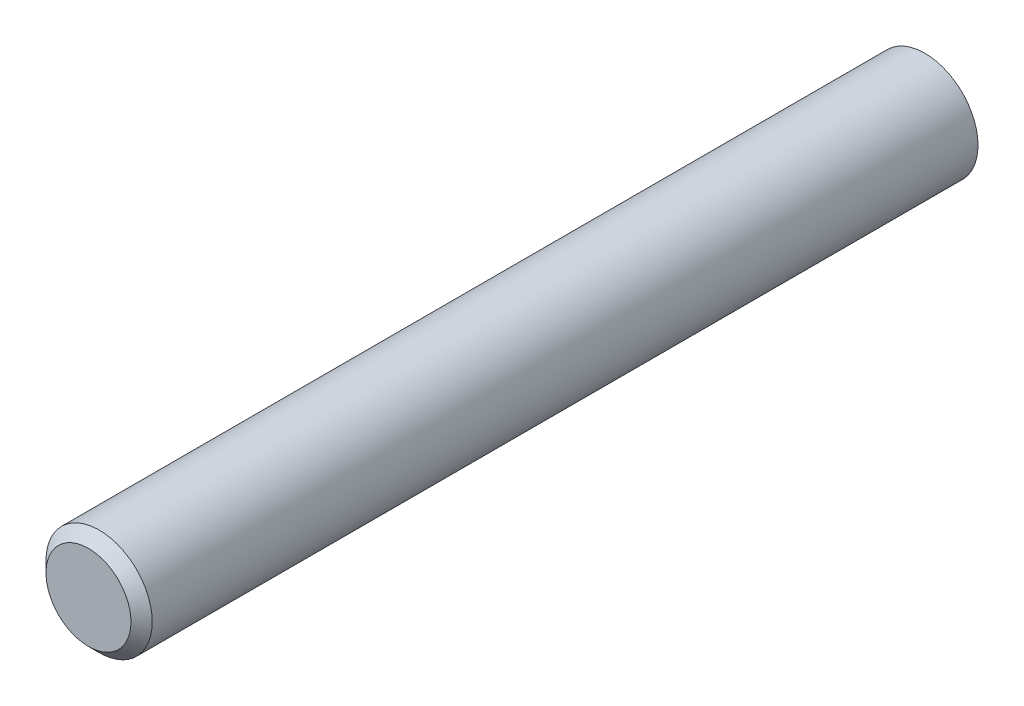
from build123d import *

# Parameters (mm, degrees)
SKETCH1_R           = 6.35
BOSS_EXTRUDE1_DEPTH = 100
CHAMFER1_SIZE       = 1.27
SCALE1_SCALE        = 2


with BuildPart() as part:
    # Sketch1 → Boss-Extrude1 (new body)
    with BuildSketch(Plane.XY):
        Circle(SKETCH1_R)
    extrude(amount=-BOSS_EXTRUDE1_DEPTH)

    # Chamfer1
    chamfer1_edges = [part.edges().sort_by_distance(p)[0] for p in [
        (-6.35, 0, 0),
    ]]
    chamfer(chamfer1_edges, length=CHAMFER1_SIZE)


with BuildPart() as part_1:
    # Scale1: scaled about (0, 0, 0)
    add(part.part.scale(SCALE1_SCALE))


solid = part_1.part
